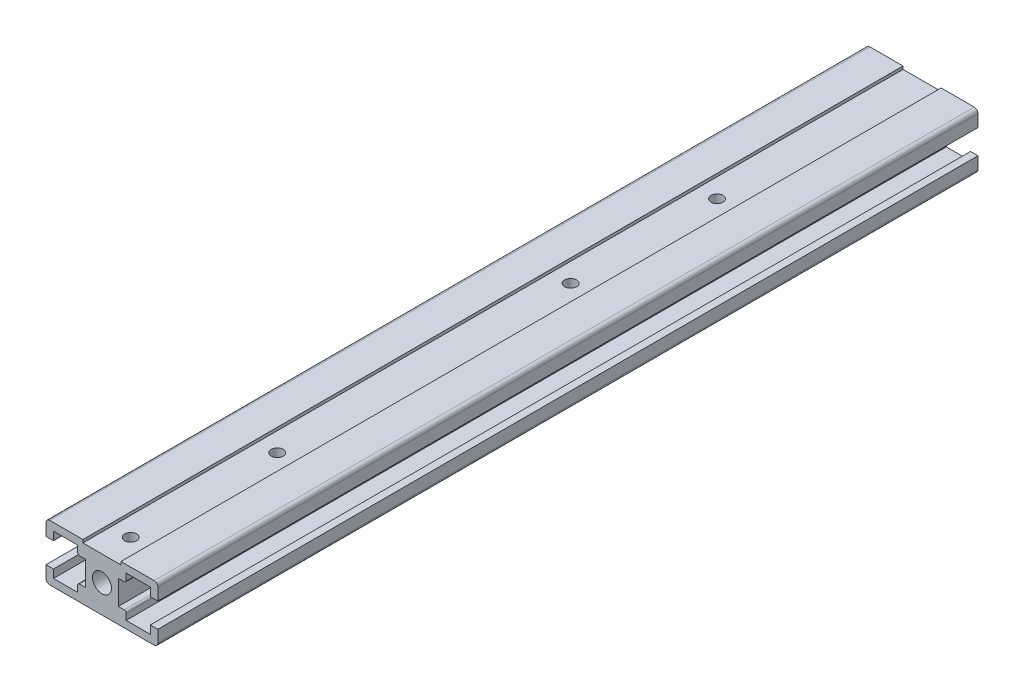
SolidWorks part; units mm, degrees
ref_plane "前视基准面" through (0, 0, 0) normal (0, 0, 1) x (1, 0, 0)
ref_plane "上视基准面" through (0, 0, 0) normal (0, 1, 0) x (1, 0, 0)
ref_plane "右视基准面" through (0, 0, 0) normal (1, 0, 0) x (0, 0, -1)
sketch "草图1" plane through (0, 0, 0) normal (0, 0, 1) x (1, 0, 0)
  line L1 (-15, 7.5) -> (15, 7.5)
  line L2 (-15, 7.5) -> (-15, -7.5)
  line L3 (-15, -7.5) -> (15, -7.5)
  line L4 (15, 7.5) -> (15, -7.5)
  line L5 (-15, 7.5) -> (15, -7.5) construction
  line L6 (-15, -7.5) -> (15, 7.5) construction
  point P0 (0, 0)
  dimension "D1" = 30
  dimension "D2" = 15
extrude "凸台-拉伸1" add sketch "草图1" along normal blind 220
fillet "圆角1" radius 1 4 edges at (15, -7.5, 110) (-15, -7.5, 110) (-15, 7.5, 110) (15, 7.5, 110)
sketch "草图2" plane through (0, 0, 220) normal (0, 0, 1) x (1, 0, 0)
  circle A0 centre (0, 0) radius 2.55
extrude "切除-拉伸1" cut sketch "草图2" against normal blind 230
sketch "草图3" plane through (0, 0, 220) normal (0, 0, 1) x (1, 0, 0)
  line L0 (-15, 6.5) -> (-15, -6.5) construction
  line L1 (-25.6, 3.25) -> (-4.4, 3.25)
  line L2 (-25.6, 3.25) -> (-25.6, -3.3)
  line L3 (-25.6, -3.3) -> (-4.4, -3.3)
  line L4 (-4.4, 3.25) -> (-4.4, -3.3)
  line L5 (-25.6, 3.25) -> (-4.4, -3.3) construction
  line L6 (-25.6, -3.3) -> (-4.4, 3.25) construction
  line L7 (14, 7.5) -> (-14, 7.5) construction
  point P0 (-15, 0)
  dimension "D1" = 6.55
  dimension "D2" = 10.6
  dimension "D3" = 4.25
extrude "切除-拉伸2" cut sketch "草图3" against normal blind 230
mirror "镜向1" about plane through (0, 0, 0) normal (1, 0, 0) of "切除-拉伸2"
sketch "草图4" plane through (0, 0, 220) normal (0, 0, 1) x (1, 0, 0)
  line L0 (-15, 6.5) -> (-15, 3.25) construction
  line L1 (-13, 5.5) -> (-6.5, 5.5)
  line L2 (-13, 5.5) -> (-13, -5.5)
  line L3 (-13, -5.5) -> (-6.5, -5.5)
  line L4 (-6.5, 5.5) -> (-6.5, -5.5)
  line L5 (14, 7.5) -> (-14, 7.5) construction
  line L6 (-14, -7.5) -> (14, -7.5) construction
  dimension "D1" = 2
  dimension "D2" = 2
  dimension "D3" = 6.5
  dimension "D4" = 2
extrude "切除-拉伸3" cut sketch "草图4" against normal blind 230
mirror "镜向2" about plane through (0, 0, 0) normal (1, 0, 0) of "切除-拉伸3"
fillet "圆角2" radius 0.5 4 edges at (-6.5, -3.3, 110) (-6.5, 3.25, 110) (6.5, -3.3, 110) (6.5, 3.25, 110)
sketch "草图5" plane through (0, 7.5, 0) normal (0, 1, 0) x (1, 0, 0)
  line L1 (14, 0) -> (-14, 0) construction
  circle A0 centre (0, -55) radius 1.6
  circle A1 centre (0, -94.2857) radius 1.6
  dimension "D1" = 3.2
  dimension "D2" = 3.2
  dimension "D4" = 55
  dimension "D3" = 39.2857
extrude "切除-拉伸4" cut sketch "草图5" against normal blind 10
pattern_linear "阵列(线性)1" count 2 spacing 118 along (0, 0, 1) of "切除-拉伸4"
sketch "草图7" plane through (0, 7.5, 0) normal (0, 1, 0) x (1, 0, 0)
  line L0 (14, 0) -> (-14, 0) construction
  line L1 (-5.1, 0) -> (5.1, 0)
  line L2 (-5.1, 0) -> (-5.1, -220)
  line L3 (-5.1, -220) -> (5.1, -220)
  line L4 (5.1, 0) -> (5.1, -220)
  line L5 (14, -220) -> (-14, -220) construction
  circle A1 centre (0, -212.2857) radius 1.6 construction
  dimension "D1" = 10.2
  dimension "D2" = 5.1
extrude "切除-拉伸6" cut sketch "草图7" against normal blind 0.8
